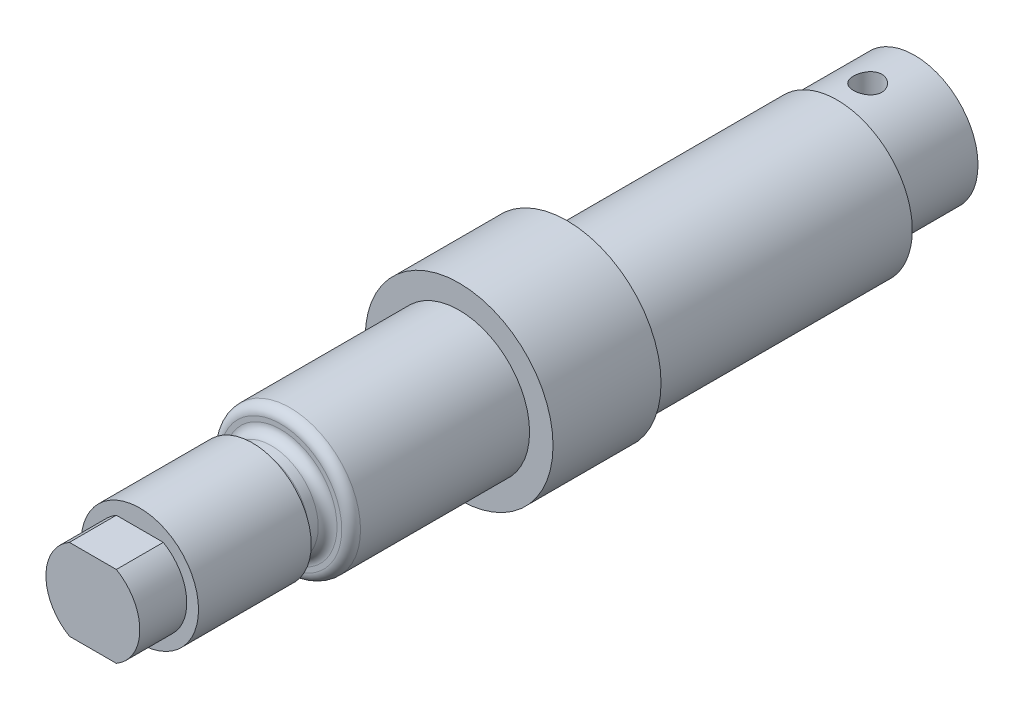
SolidWorks part; units mm, degrees
material "45"
ref_plane "Front" through (0, 0, 0) normal (0, 0, 1) x (1, 0, 0)
ref_plane "Top" through (0, 0, 0) normal (0, 1, 0) x (1, 0, 0)
ref_plane "Right" through (0, 0, 0) normal (1, 0, 0) x (0, 0, -1)
sketch "Sketch2" plane through (0, 0, 0) normal (0, 0, 1) x (1, 0, 0)
  circle A0 centre (0, 0) radius 13.5
  dimension "D1" = 27
extrude "Extrude1" add sketch "Sketch2" along normal blind 19
sketch "Sketch3" plane through (0, 0, 19) normal (0, 0, 1) x (1, 0, 0)
  line L0 (0, 0) -> (14.4038, 0) construction
  circle A0 centre (2.5, 0) radius 16
  circle A1 centre (0, 0) radius 13.5 construction
  dimension "D1" = 32
  dimension "D2" = 2.5
extrude "Extrude2" add sketch "Sketch3" along normal blind 55
sketch "Sketch4" plane through (0, 0, 74) normal (0, 0, 1) x (1, 0, 0)
  line L0 (0, 0) -> (-21.1817, 0) construction
  circle A0 centre (0, 0) radius 20
  dimension "D1" = 40
extrude "Extrude3" add sketch "Sketch4" along normal blind 23
sketch "Sketch5" plane through (0, 0, 97) normal (0, 0, 1) x (1, 0, 0)
  circle A0 centre (0, 0) radius 15
  dimension "D1" = 30
extrude "Extrude4" add sketch "Sketch5" along normal blind 38
sketch "Sketch6" plane through (0, 0, 135) normal (0, 0, 1) x (1, 0, 0)
  circle A0 centre (0, 0) radius 10
  dimension "D1" = 20
extrude "Extrude5" add sketch "Sketch6" along normal blind 6
sketch "Sketch7" plane through (0, 0, 141) normal (0, 0, 1) x (1, 0, 0)
  circle A0 centre (0, 0) radius 12.5
  dimension "D1" = 25
extrude "Extrude6" add sketch "Sketch7" along normal blind 24
cosmetic thread "Cosmetic Thread1" parameters "D2"=23
sketch "Sketch8" plane through (0, 0, 165) normal (0, 0, 1) x (1, 0, 0)
  line L0 (-5, 8.6603) -> (5, 8.6603)
  line L1 (0, 7.1489) -> (0, -14.6517) construction
  line L2 (-5, -8.6603) -> (5, -8.6603)
  line L3 (-22.3845, 0) -> (25.905, 0) construction
  arc A0 (-5, 8.6603) -> (-5, -8.6603) centre (0, 0) ccw
  arc A1 (5, -8.6603) -> (5, 8.6603) centre (0, 0) ccw
  dimension "D1" = 20
  dimension "D2" = 10
extrude "Extrude7" add sketch "Sketch8" along normal blind 10
sketch "Sketch9" plane through (0, 0, 0) normal (0, 1, 0) x (1, 0, 0)
  circle A0 centre (0, -10) radius 3
  dimension "D1" = 6
  dimension "D2" = 10
extrude "Cut-Extrude1" cut sketch "Sketch9" against normal mid plane 30
chamfer "Chamfer1" [suppressed] distance 2 angle 45
sketch "Sketch10" plane through (0, 0, 74) normal (0, 0, -1) x (-1, 0, 0)
  line L0 (-9.6825, 17.5) -> (9.6825, 17.5)
  line L1 (-9.6825, -17.5) -> (9.6825, -17.5)
  line L2 (-25.9259, 0) -> (24.2861, 0) construction
  circle A0 centre (0, 0) radius 20 construction
  arc A1 (-9.6825, -17.5) -> (9.6825, -17.5) centre (0, 0) ccw
  arc A2 (9.6825, 17.5) -> (-9.6825, 17.5) centre (0, 0) ccw
  dimension "D1" = 35
extrude "Cut-Extrude2" [suppressed] cut sketch "Sketch10" against normal up to next
chamfer "Chamfer2" [suppressed] distance 1 angle 45
fillet "Fillet1" radius 2 3 edges at (10, 0, 135) (10, 0, 141) (15, 0, 135)
